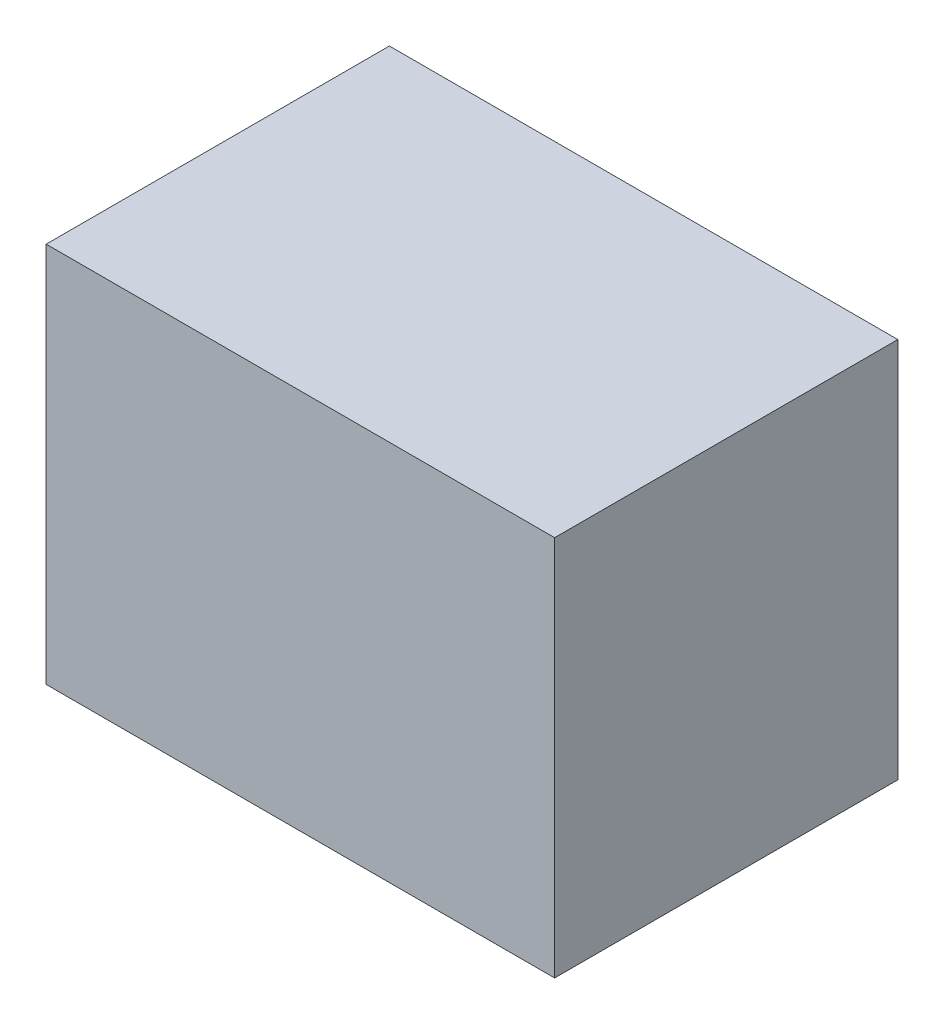
SolidWorks part; units mm, degrees
material "1023 Carbon Steel Plate (SS)"
ref_plane "Front Plane" through (0, 0, 0) normal (0, 0, 1) x (1, 0, 0)
ref_plane "Top Plane" through (0, 0, 0) normal (0, 1, 0) x (1, 0, 0)
ref_plane "Right Plane" through (0, 0, 0) normal (1, 0, 0) x (0, 0, -1)
sketch "Sketch1" plane through (0, 0, 0) normal (0, 0, 1) x (1, 0, 0)
  line L1 (20, 15) -> (-20, 15)
  line L2 (20, 15) -> (20, -15)
  line L3 (20, -15) -> (-20, -15)
  line L4 (-20, 15) -> (-20, -15)
  line L5 (20, 15) -> (-20, -15) construction
  line L6 (20, -15) -> (-20, 15) construction
  point P0 (0, 0)
  dimension "D1" = 40
  dimension "D2" = 30
extrude "Boss-Extrude1" add sketch "Sketch1" along normal blind 27
